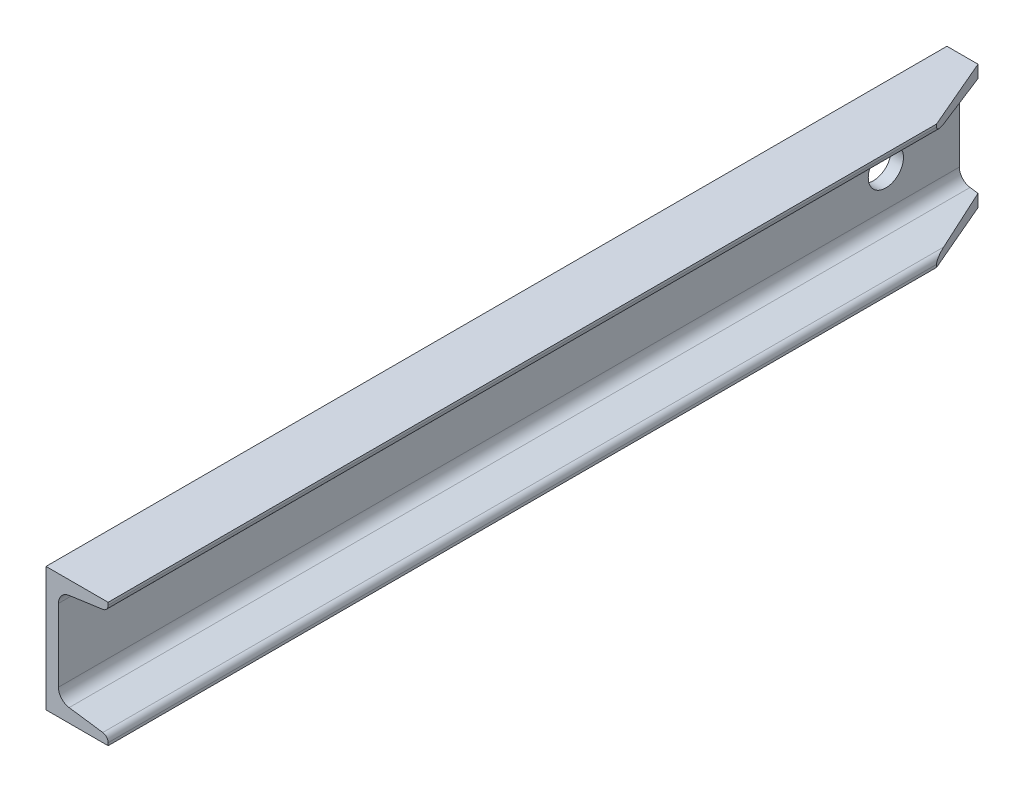
from build123d import *

# Parameters (mm, degrees)
BOSS_EXTRUDE1_DEPTH = 435
SKETCH2_R           = 8.5
CUT_EXTRUDE1_DEPTH  = 435
CUT_EXTRUDE2_DEPTH  = 435


with BuildPart() as part:
    # Sketch1 → Boss-Extrude1 (new body)
    with BuildSketch(Plane.XY):
        with BuildLine():
            Line((0, 0), (-30, 0))
            Line((-30, 0), (-30, -60))
            Line((-30, -60), (0, -60))
            Line((0, -60), (0, -58.715972734))
            ThreePointArc((0, -58.715972734), (-0.735871259, -56.747795647), (-2.582480697, -55.745168528))
            Line((-2.582480697, -55.745168528), (-18.835038606, -53.461020473))
            ThreePointArc((-18.835038606, -53.461020473), (-22.528257481, -51.455766235), (-24, -47.519412061))
            Line((-24, -47.519412061), (-24, -12.480587939))
            ThreePointArc((-24, -12.480587939), (-22.528257481, -8.544233765), (-18.835038606, -6.538979527))
            Line((-18.835038606, -6.538979527), (-2.582480697, -4.254831472))
            ThreePointArc((-2.582480697, -4.254831472), (-0.735871259, -3.252204353), (0, -1.284027266))
            Line((0, -1.284027266), (0, 0))
        make_face()
    extrude(amount=BOSS_EXTRUDE1_DEPTH)

    # Sketch2 → Cut-Extrude1 (cut)
    with BuildSketch(Plane.ZY.offset(30)):
        with Locations(Location((35.5, -30, 0), (0, 0, 270))):
            Circle(SKETCH2_R)
    extrude(amount=-CUT_EXTRUDE1_DEPTH, mode=Mode.SUBTRACT)

    # Sketch3 → Cut-Extrude2 (cut)
    with BuildSketch(Plane(origin=(0, 0, 0), x_dir=(1, 0, 0), z_dir=(0, 1, 0))):
        Polygon((-15, 0), (0, 0), (0, -35), align=None)
    extrude(amount=-CUT_EXTRUDE2_DEPTH, mode=Mode.SUBTRACT)


solid = part.part
